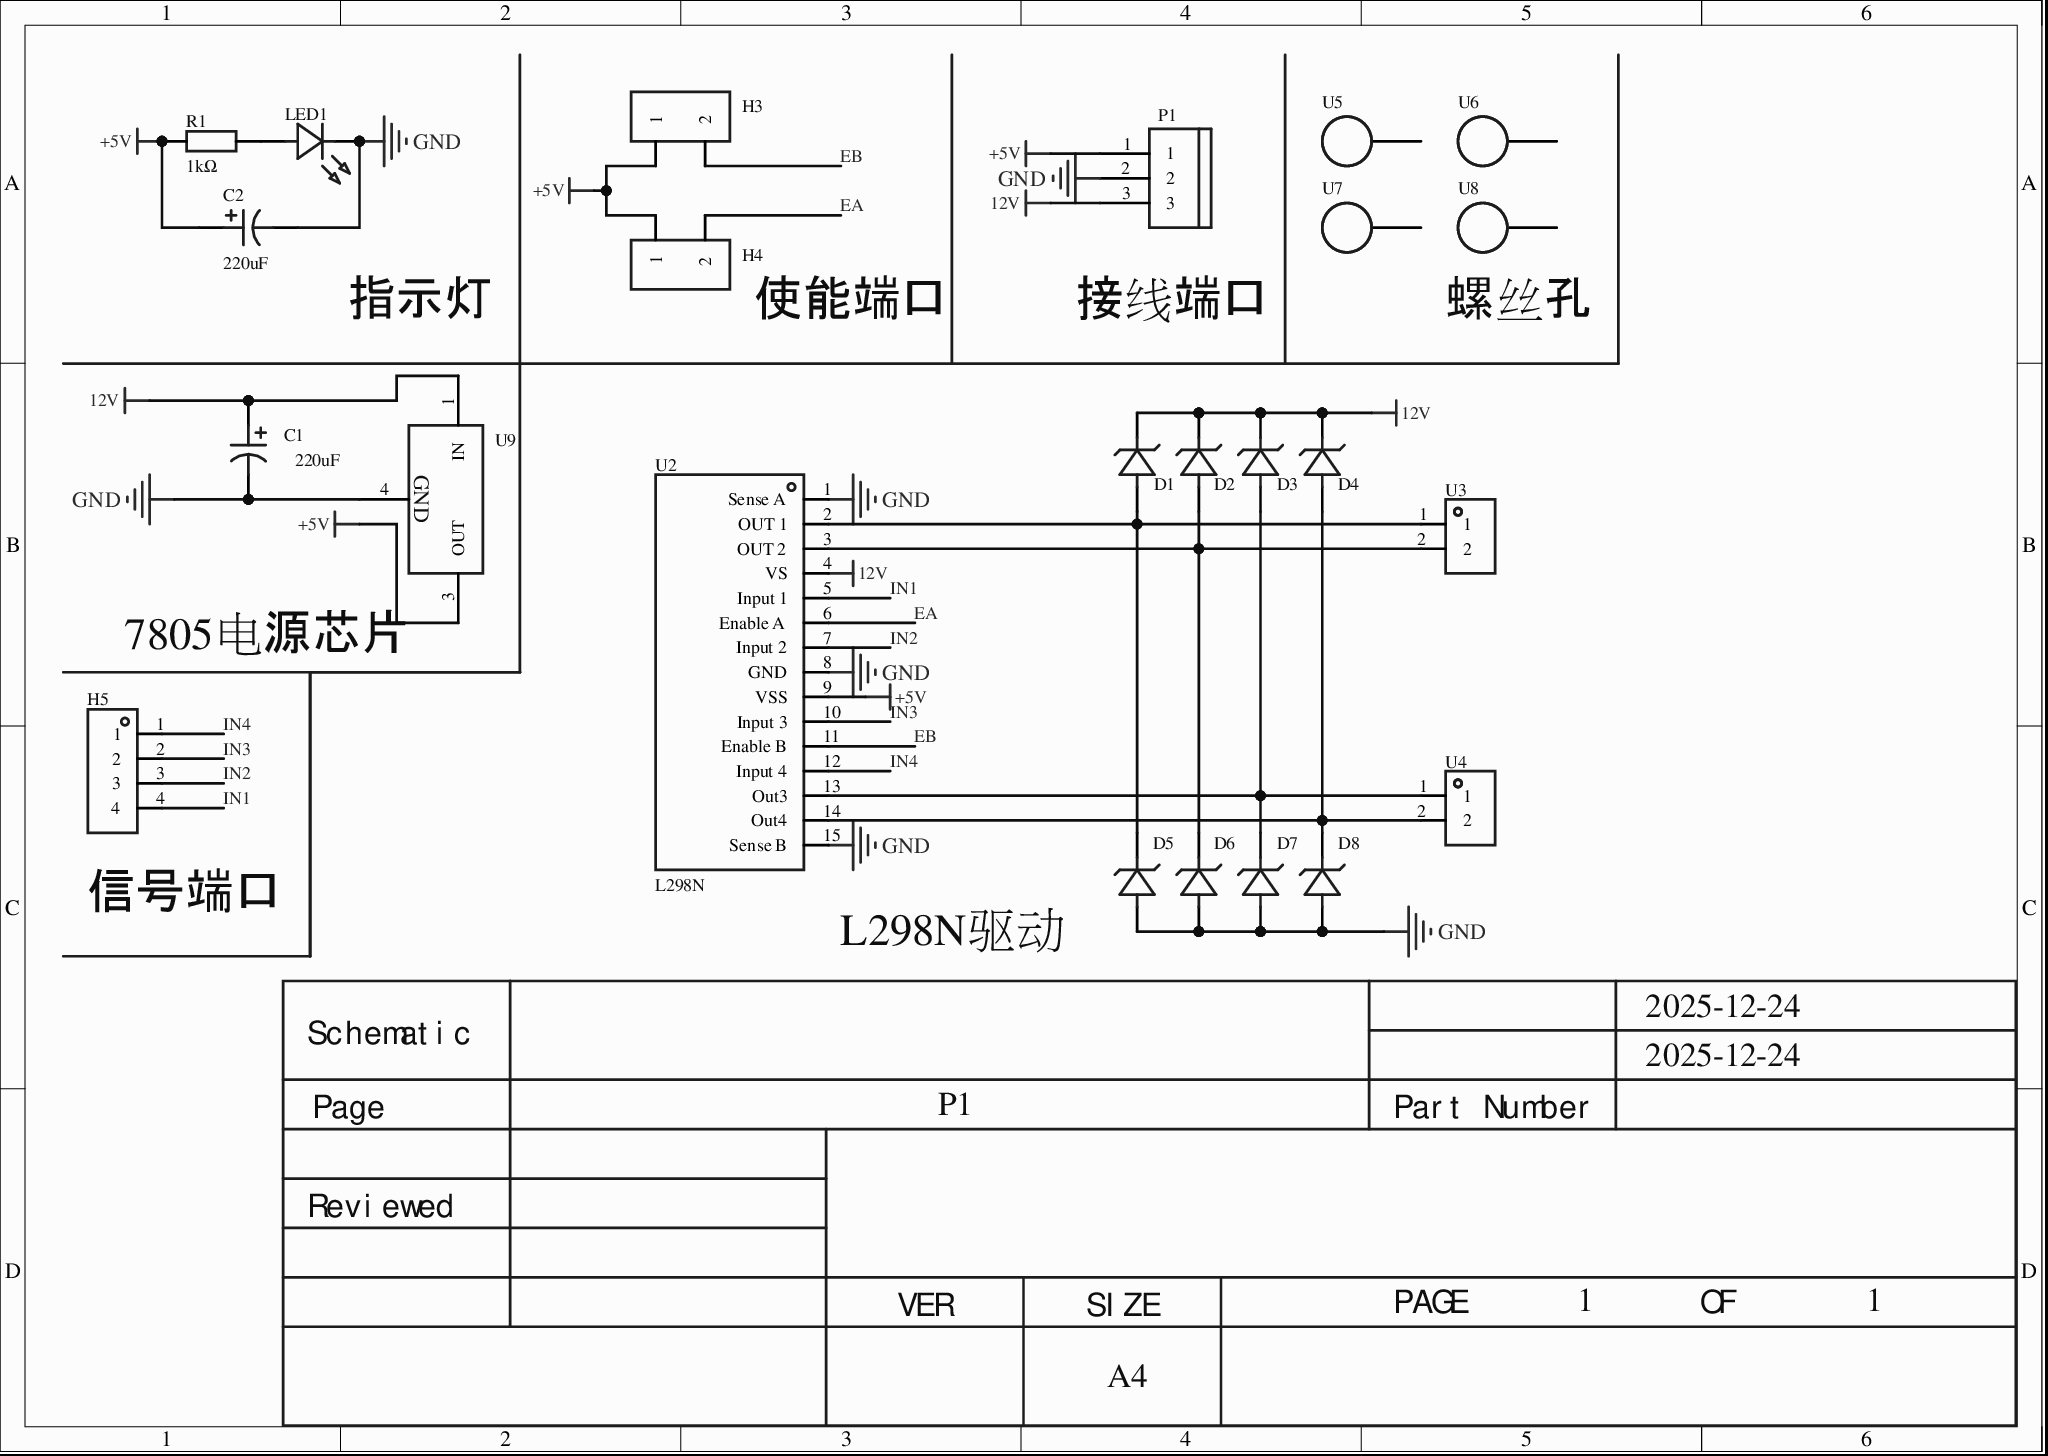
[diagram p0: MISC51599-3.schdoc]
# Altium project MISC51599-2.PrjPcb
1 sheet, 24 parts. Net scope: global (net labels, ports and power ports of the same name join across sheets).
Board file: MISC51599.pcbdoc

## Sheet MISC51599-3.schdoc
size 210 x 149 mm; Version: V1.0; @Project Name: MISC51599; @Page Count: 1; @Update Date: 2025-12-24; @Create Date: 2025-12-24; @Schematic Name: MISC51599; @Page No: 1

### Parts
C1  value 220uF  [CAP-SMD_BD8.0-L8.3-W8.3-LS9.3-FD]
C2  value 220uF  [CAP-SMD_BD8.0-L8.3-W8.3-LS9.3-FD]
D1  (no value)  [SOD-123FL_L2.7-W1.8-LS3.8-RD]
D2  (no value)  [SOD-123FL_L2.7-W1.8-LS3.8-RD]
D3  (no value)  [SOD-123FL_L2.7-W1.8-LS3.8-RD]
D4  (no value)  [SOD-123FL_L2.7-W1.8-LS3.8-RD]
D5  (no value)  [SOD-123FL_L2.7-W1.8-LS3.8-RD]
D6  (no value)  [SOD-123FL_L2.7-W1.8-LS3.8-RD]
D7  (no value)  [SOD-123FL_L2.7-W1.8-LS3.8-RD]
D8  (no value)  [SOD-123FL_L2.7-W1.8-LS3.8-RD]
H3  (no value)  [HDR-TH_2P-P2.54-V-M-1]
H4  (no value)  [HDR-TH_2P-P2.54-V-M-1]
H5  826629-4  [HDR-TH_4P-P2.54-V-M-1]  (value not drawn)
LED1  (no value)  [LED0805-RD_BLUE]
P1  (no value)  [CONN-TH_3P-P5.00_WJ500V-5.08-3P]
R1  value 1kΩ  [R0805]
U2  L298N  [MULTIWATT-15_L19.6-W5.0-P1.27-L]
U3  (no value)  [CONN-TH_DB302-5.0-2P]
U4  (no value)  [CONN-TH_DB302-5.0-2P]
U5  (no value)  [SMD_BD4.2-L4.7-W4.7-D3.0]
U6  (no value)  [SMD_BD4.2-L4.7-W4.7-D3.0]
U7  (no value)  [SMD_BD4.2-L4.7-W4.7-D3.0]
U8  (no value)  [SMD_BD4.2-L4.7-W4.7-D3.0]
U9  L78M05ABDT-TR  [TO-252-2_L6.5-W6.1-P4.58-LS10.0-TL]  (value not drawn)

### Nets
12V: C1.1 D1.1(K) D2.1(K) D3.1(K) D4.1(K) P1.3 U2.4(VS) U9.1(IN)
+5V: C2.1 H3.1 H4.1 P1.1 R1.2 U2.9(VSS) U9.3(OUT)
GND: C1.2 C2.2 D5.2(A) D6.2(A) D7.2(A) D8.2(A) LED1.1(K) P1.2 U2.1(Sense_A) U2.8(GND) U2.15(Sense_B) U9.4(GND)
EA: H4.2 U2.6(Enable_A)
EB: H3.2 U2.11(Enable_B)
IN1: H5.4 U2.5(Input_1)
IN2: H5.3 U2.7(Input_2)
IN3: H5.2 U2.10(Input_3)
IN4: H5.1 U2.12(Input_4)
NetD1_2: D1.2(A) D5.1(K) U2.2(OUT_1) U3.1
NetD2_2: D2.2(A) D6.1(K) U2.3(OUT_2) U3.2
NetD3_2: D3.2(A) D7.1(K) U2.13(Out3) U4.1
NetD4_2: D4.2(A) D8.1(K) U2.14(Out4) U4.2
NetLED1_2: LED1.2(A) R1.1

Not connected (* = marked no-connect by the designer): U5 1; U6 1; U7 1; U8 1

### Notes on the sheet
- 指示灯
- (near H4) 使能端口
- 接线端口
- (near U8) 螺丝孔
- 7805电源芯片
- (near H5) 信号端口
- (near U2) L298N驱动
- 2025-12-24
- Schematic
- Page
- P1
- Part Number
- Reviewed
- VER
- SIZE
- A4
- PAGE
- 1
- OF

### Library data of the parts
C1 C2 = EMK1VM221FB0D00R: 容值:220uF;精度:±20%;额定电压:35V;电容体直径:-;电容体长度:-;纹波电流:-;等效串联电阻:-;工作寿命:-;工作温度:-;; Manufacturer: AISHI(艾华集团); AddInBom: yes; ModelId: ae37c166a99f49b1b935231edf05d58d; ModelTransform: 366.1,326.8,0,0,0,0,0,0,0; Tolerance: ±20%; Rated Voltage: 35V; Device: EMK1VM221FB0D00R; Symbol: EMK1VM221FB0D00R; LCSC Part Name: 220uF ±20% 35V; SupplierPart: C724731; ManufacturerPart: EMK1VM221FB0D00R; Supplier Footprint: SMD,8x10.5mm; JLCPCB Part Class: Extended Part; Datasheet: https://atta.szlcsc.com/upload/public/pdf/source/20200818/C724731_E3C3C738DF50876976EE53B5D20E1717.pdf; Supplier: LCSC; ConvertToPcb: yes; FootprintName: CAP-SMD_BD8.0-L8.3-W8.3-LS9.3-FD; ModelName: CAP-SMD_BD8.0-L8.3-W8.3-LS9.3-FD; φD: -; L: -; Ripple Current: -; Equivalent Series Resistance(ESR): -; Lifetime @ Temp: -; Operating Temperature: -
D1-D8 = 1N4007: 二极管配置:独立式;直流反向耐压(Vr):1kV;平均整流电流(Io):1A;正向压降(Vf):1.1V@1A;反向电流(Ir):10A@1kV;; Manufacturer: TWGMC(台湾迪嘉); Symbol: 1N4007_C727082; AddInBom: yes; ModelId: 86f9151e155e4fe2af0c4f2e0a80302e; ModelName: SOD-123FL_L2.8-W1.8-H1.1-LS3.6; ModelTransform: 141.7,70.9,0,180,0,0,0,0,0; Diode Configuration: 独立式; Reverse Voltage (Vr): 1kV; Average Rectified Current (Io): 1A; Reverse Leakage Current: 10A@1kV; Device: 1N4007; LCSC Part Name: 1kV 1A 1.1V@1A; SupplierPart: C727082; ManufacturerPart: 1N4007; Supplier Footprint: SOD-123FL; JLCPCB Part Class: Extended Part; Datasheet: https://atta.szlcsc.com/upload/public/pdf/source/20200828/C727082_2F914037E829F0E2238583225D7ED281.pdf; Supplier: LCSC; ConvertToPcb: yes; FootprintName: SOD-123FL_L2.7-W1.8-LS3.8-RD; Forward Voltage (Vf@If): 1.1V@1A
H3 H4 = 826629-2: 间距:2.54mm;总PIN位数:2;排数:1;插针结构:-;行距:-;安装类型:直插;圆针/方针:-;额定电流:-;额定电压:-;配合针长度:-;塑高:-;触头材质:黄铜;触头镀层:-;颜色:绿色;; Manufacturer: TE Connectivity(美国泰科); Symbol: Header-Male-2.54_1x2; AddInBom: yes; ModelId: 79b2e9f2d70a4d68a1b7098f27c6d4c5; ModelName: HDR-M-2.54_1x2; ModelTransform: 200,100,0,0,0,0,0,0,-118.11; Pitch: 2.54mm; Device: 826629-2; LCSC Part Name: 2.54mm 分离式  金; SupplierPart: C86471; ManufacturerPart: 826629-2; Supplier Footprint: 插件; JLCPCB Part Class: Extended Part; Datasheet: https://atta.szlcsc.com/upload/public/pdf/source/20161105/1478330325829.pdf; Supplier: LCSC; ConvertToPcb: yes; FootprintName: HDR-TH_2P-P2.54-V-M-1; Number of Pins: 2; Number of Rows: 1; Pin Structure: -; Row Spacing: -; Mounting Type: 直插; Circluar Pins/Square Pins: -; Current Rating (Max): -; Voltage Rating (Max): -; Length of Mating Pin: -; Insulation Height: -; Contact Material: 黄铜; Contact Plating: -; Color: 绿色
H5 = 826629-4: 排数:单排;总PIN位数:4;间距:2.54mm;插针结构:1x4P;行距:-;安装类型:直插;圆针/方针:-;额定电流:-;额定电压:-;配合针长度:6.7mm;塑高:2.8mm;端接针长度:3.2mm;触头材质:-;工作温度范围:-;颜色:绿色;; Manufacturer: TE Connectivity(美国泰科); AddInBom: yes; ModelId: f8e5d153169943fabcf3383e1c9553c6; ModelName: HDR-M-2.54_1x4; ModelTransform: 399.999,100,0,0,0,0,0,0,-118.11; Pitch: 2.54mm; Pin Structure: 1x4P; Device: 826629-4; Symbol: 826629-4; LCSC Part Name: 2.54mm 1x4P 直插; SupplierPart: C590277; ManufacturerPart: 826629-4; Supplier Footprint: 插件,P=2.54mm; JLCPCB Part Class: Extended Part; Datasheet: https://atta.szlcsc.com/upload/public/pdf/source/20210923/FCC8CD9A04BA2624CF68C067B4A5B53A.pdf; Supplier: LCSC; ConvertToPcb: yes; FootprintName: HDR-TH_4P-P2.54-V-M-1; Number of Rows: 单排; Number of Pins: 4; Row Spacing: -; Mounting Type: 直插; Circluar Pins/Square Pins: -; Current Rating (Max): -; Voltage Rating (Max): -; Length of Mating Pin: 6.7mm; Insulation Height: 2.8mm; Length of End Connection Pin: 3.2mm; Contact Material: -; Operating Temperature Range: -; Color: 绿色
LED1 = RF-BGB170TS-CB-E0: 发光颜色:蓝灯;二极管配置:-;透镜颜色:-;主波长:-;峰值波长:-;色温:-;光通量(25时):-;测试电流:20mA;正向电压(VF):-;发光强度:-;功率:70mW;发光角度:140°;安装方式:正贴;工作温度:-40~+85;; Manufacturer: Refond(瑞丰); AddInBom: yes; ModelId: b1c5ed7a4f6e46d3bc6f6cc7c20f3fea; ModelName: LED0805-RD; ModelTransform: 79.5,49.2,0,0,0,0,0,0,0; Emitted Color: 蓝灯; Forward Current: 20mA; Power Dissipation: 70mW; Viewing Angle: 140°; Mounting Sytle: 正贴; Operating Temperature: -40~+85; Device: RF-BGB170TS-CB-E0; Symbol: RF-BGB170TS-CB-E0; LCSC Part Name: 蓝灯 正贴; SupplierPart: C2908306; ManufacturerPart: RF-BGB170TS-CB-E0; Supplier Footprint: 0805; JLCPCB Part Class: Extended Part; Datasheet: https://atta.szlcsc.com/upload/public/pdf/source/20211101/C871A18E9B6E101B84BDF0C661245F86.pdf; Supplier: LCSC; ConvertToPcb: yes; FootprintName: LED0805-RD_BLUE; Diode Configuration: -; Lens Color: -; Dominant Wavelength: -; Peak Wavelength: -; Color Temperature: -; Luminous Flux (@25℃): -; Forward Voltage (VF): -; Luminous Intensity: -
P1 = WJ500V-5.08-3P: 间距:5.08mm;排数:1;每排PIN数:3;安装方式:直针;额定电流:18A;额定电压:250V;线规 - AWG:14~30;线规 - mm?:2.5;工作温度范围:-40~+105;颜色:绿色;; Manufacturer: KANGNEX(康奈克斯电气); Symbol: WJ500V-5.08-3P-14-00A; AddInBom: yes; ModelId: f80d5090781743d49abcb05979f5618f; ModelName: CONN-TH_3P_L15.3-W10.2-P5.08; ModelTransform: 619.7,413.4,0,180,0,0,7.9,0,-157.5; Pitch: 5.08mm; Number of PINs Per Row: 3; Current Rating (Max): 18A; Voltage Rating (Max): 250V; Wire Gauge - AWG: 14~30; Wire Gauge - mm?: 2.5; Operating Temperature Range: -40~+105; Device: WJ500V-5.08-3P; LCSC Part Name: 5.08mm 排数:1 每排P数:3 直针 可拼接; SupplierPart: C72334; ManufacturerPart: WJ500V-5.08-3P; Supplier Footprint: P=5.08mm; JLCPCB Part Class: Extended Part; Datasheet: https://atta.szlcsc.com/upload/public/pdf/source/20191225/C72334_8A5EF831D67650233B6B1E3F2BC06274.pdf; Supplier: LCSC; ConvertToPcb: yes; FootprintName: CONN-TH_3P-P5.00_WJ500V-5.08-3P; Number of Rows: 1; Mounting Style: 直针; Color: 绿色
R1 = RS-05K102JT: 阻值:1kΩ;精度:±5%;功率:125mW;温度系数:±100ppm/;最大工作电压:150V;工作温度范围:-55~+155;; Manufacturer: FH(风华); AddInBom: yes; ModelId: 37a81e68749a4138bd2dfa6897b24b85; ModelName: R0805_L2.0-W1.3-H0.6; ModelTransform: 78.74,51.181,0,0,0,0,0,-0.0005,0; Tolerance: ±5%; Power(Watts): 125mW; Overload Voltage (Max): 150V; Temperature Coefficient: ±100ppm/; Operating Temperature Range: -55~+155; Device: RS-05K102JT; Symbol: RS-05K102JT; LCSC Part Name: 1kΩ ±5%; SupplierPart: C115302; ManufacturerPart: RS-05K102JT; Supplier Footprint: 0805; JLCPCB Part Class: Extended Part; Datasheet: https://atta.szlcsc.com/upload/public/pdf/source/20170704/1499151304704.pdf; Supplier: LCSC; ConvertToPcb: yes; FootprintName: R0805
U2 = L298N_C19922: 电源电压:4.5V~7V;特性:过流保护(OCP)；过热保护(OPT);; Manufacturer: ST(意法半导体); AddInBom: yes; ModelId: 17dbda3c803a45a0ac2c74e6ab5d5790; ModelTransform: 795.27392,389.3693,0,0,0,0,0,84.646,-137.795; Device: L298N_C19922; Symbol: L298N_C19922; LCSC Part Name: L298N; SupplierPart: C19922; ManufacturerPart: L298N; Supplier Footprint: Multiwatt-15-V; JLCPCB Part Class: Extended Part; Datasheet: https://atta.szlcsc.com/upload/public/pdf/source/20131014/1457706655076.pdf; Supplier: LCSC; ConvertToPcb: yes; FootprintName: MULTIWATT-15_L19.6-W5.0-P1.27-L; ModelName: MULTIWATT-15_L19.6-W5.0-P1.27-L; Supply Voltage: 4.5V~7V; Feature: 过流保护(OCP)；过热保护(OPT); Operating Temperature: -40℃~+150℃@(Tj)
U3 U4 = DB302-5.0-2P-GN-S: Manufacturer: DIBO(地博电气); AddInBom: yes; ModelId: af2d1fe21b58404e908b9acd6fb20001; ModelTransform: 427.9519,354.33,0,0,0,0,16.727,0.827,-157.48; Device: DB302-5.0-2P-GN-S; Symbol: DB302-5.0-2P-GN-S; LCSC Part Name: 2P P=5mm; SupplierPart: C2997275; ManufacturerPart: DB302-5.0-2P-GN-S; Supplier Footprint: P=5mm; JLCPCB Part Class: Extended Part; Datasheet: https://atta.szlcsc.com/upload/public/pdf/source/20220418/F63E4822E301FF035E2D9136E480A4B5.pdf; Supplier: LCSC; ConvertToPcb: yes; FootprintName: CONN-TH_DB302-5.0-2P; ModelName: CONN-TH_DB302-5.0-2P
U5-U8 = 铜柱M3*5+6: 螺柱类型:单通螺柱;公称直径:M3;螺距:-;长度:11mm;执行标准:-;强度等级:-;材料:-;表面处理:-;; Manufacturer: 国产; AddInBom: yes; Bolts Type: 单通螺柱; Device: 铜柱M3*5+6; Symbol: 铜柱M3*5+6; LCSC Part Name: 铜柱M3*5+6; SupplierPart: C87703; ManufacturerPart: 铜柱M3*5+6; Supplier Footprint: M3*5+6; JLCPCB Part Class: Extended Part; Datasheet: https://atta.szlcsc.com/upload/public/pdf/source/20180629/C87703_D0202CF0C285C70F41F1E6F27424EC8C.pdf; Supplier: LCSC; ConvertToPcb: yes; FootprintName: SMD_BD4.2-L4.7-W4.7-D3.0; Nominal Diameter: M3; Pitch of Thread: -; Length: 11mm; Standard: -; Nut Performance Class: -; Material: -; Finish: -
U9 = L78M05ABDT-TR: L78M Series 500 mA 5 V Three Terminal Positive Voltage LDO Regulator - TO-252; Manufacturer: ST(意法半导体); AddInBom: yes; ModelId: 6b2ea0154a284e6db98f69bccdba3606; ModelName: TO-252-2_L6.5-W6.1-H2.3-LS10.0-P4.58; ModelTransform: 255.905,390.52442,0,270,0,0,38.183,0.432,0; Device: L78M05ABDT-TR; Symbol: L78M05ABDT-TR; LCSC Part Name: L78M05ABDT-TR; SupplierPart: C58069; ManufacturerPart: L78M05ABDT-TR; Supplier Footprint: TO-252-2(DPAK); JLCPCB Part Class: Basic Part; Datasheet: https://atta.szlcsc.com/upload/public/pdf/source/20150912/1457707362652.pdf; Supplier: LCSC; ConvertToPcb: yes; FootprintName: TO-252-2_L6.5-W6.1-P4.58-LS10.0-TL